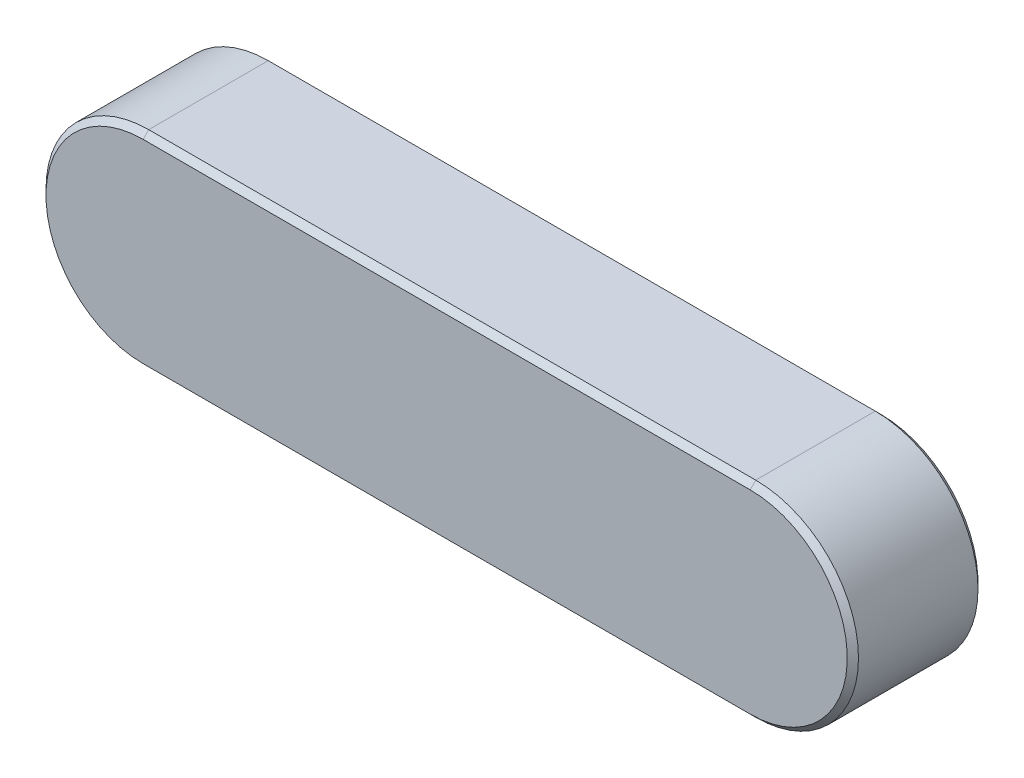
from build123d import *

# Parameters (mm, degrees)
BOSS_EXTRUDE1_DEPTH = 7
CHAMFER1_SIZE       = 0.6


with BuildPart() as part:
    # Sketch1 → Boss-Extrude1 (new, symmetric)
    with BuildSketch(Plane.XY):
        with BuildLine():
            Line((-26.425596314, 14.36924081), (38.574403686, 14.36924081))
            ThreePointArc((38.574403686, 14.36924081), (49.574403686, 3.36924081), (38.574403686, -7.63075919))
            Line((38.574403686, -7.63075919), (-26.425596314, -7.63075919))
            ThreePointArc((-26.425596314, -7.63075919), (-37.425596314, 3.36924081), (-26.425596314, 14.36924081))
        make_face()
    extrude(amount=BOSS_EXTRUDE1_DEPTH, both=True)

    # Chamfer1
    chamfer1_edges = [part.edges().sort_by_distance(p)[0] for p in [
        (49.574403686, 3.36924081, 7),
        (6.074403686, 14.36924081, 7),
        (-37.425596314, 3.36924081, 7),
        (6.074403686, 14.36924081, -7),
        (49.574403686, 3.36924081, -7),
        (6.074403686, -7.63075919, -7),
        (-37.425596314, 3.36924081, -7),
        (6.074403686, -7.63075919, 7),
    ]]
    chamfer(chamfer1_edges, length=CHAMFER1_SIZE)


solid = part.part
